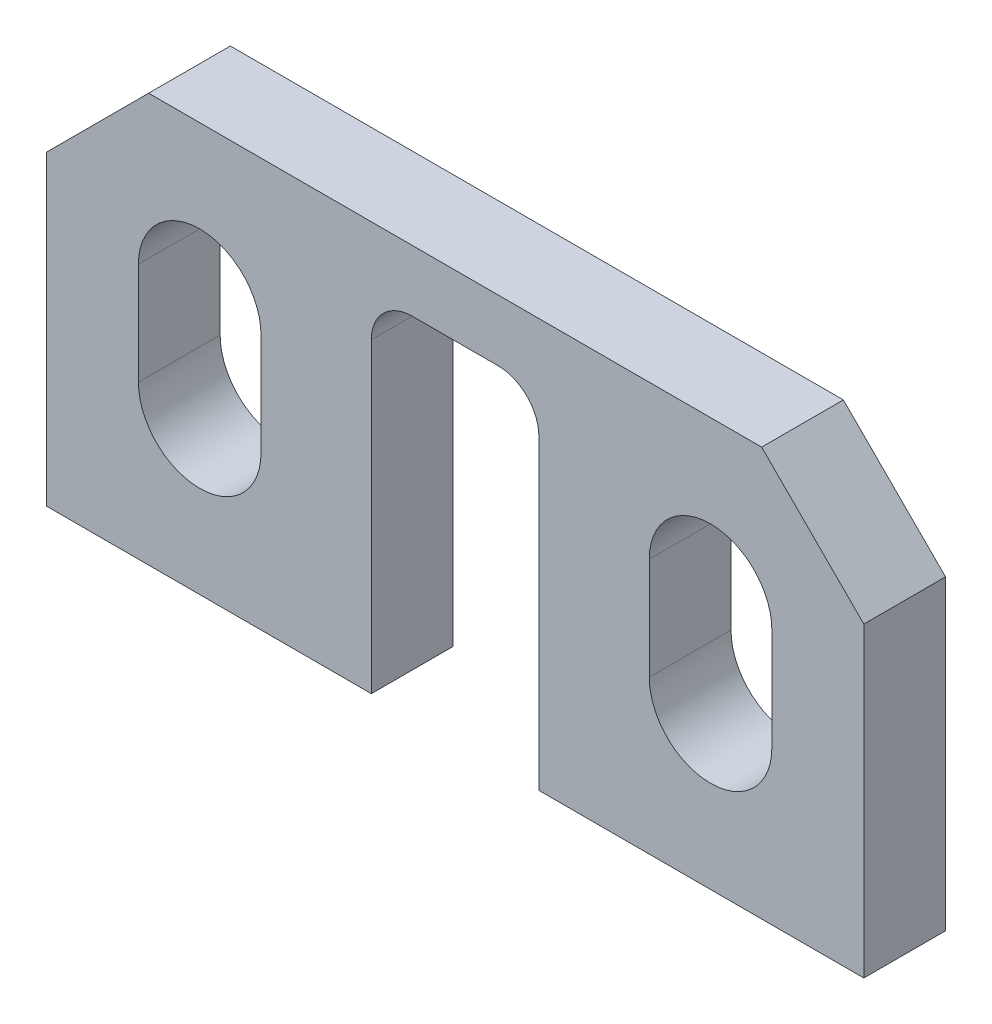
SolidWorks part; units mm, degrees
ref_plane "前视基准面" through (0, 0, 0) normal (0, 0, 1) x (1, 0, 0)
ref_plane "上视基准面" through (0, 0, 0) normal (0, 1, 0) x (1, 0, 0)
ref_plane "右视基准面" through (0, 0, 0) normal (1, 0, 0) x (0, 0, -1)
sketch "草图1" plane through (0, 0, 0) normal (0, 0, 1) x (1, 0, 0)
  line L0 (0, 10) -> (0, 0) construction
  line L1 (-20, 10) -> (20, 10)
  line L2 (-20, 10) -> (-20, -10)
  line L3 (-20, -10) -> (20, -10)
  line L4 (20, 10) -> (20, -10)
  line L5 (0, 0) -> (20, 0) construction
  dimension "D1" = 40
  dimension "D2" = 20
extrude "凸台-拉伸1" add sketch "草图1" along normal blind 4
sketch "草图2" plane through (0, 0, 4) normal (0, 0, 1) x (1, 0, 0)
  line L0 (0, 7) -> (0, -18.9473) construction
  line L1 (4.1, 7) -> (4.1, -18.9473)
  line L2 (-4.1, 7) -> (-4.1, -18.9473)
  line L3 (20, 10) -> (-20, 10) construction
  line L4 (-4.1, 7) -> (4.1, 7)
  arc A1 (-4.1, -18.9473) -> (4.1, -18.9473) centre (0, -18.9473) ccw
  point P3 (0, -7.9736)
  dimension "D1" = 8.2
  dimension "D2" = 3
extrude "切除-拉伸1" cut sketch "草图2" against normal through all
chamfer "倒角1" distance 5 angle 45 2 edges at (20, 10, 2) (-20, 10, 2)
sketch "草图3" plane through (0, 0, 4) normal (0, 0, 1) x (1, 0, 0)
  line L0 (0, 15.5999) -> (0, 0) construction
  line L1 (0, 0) -> (25, 0) construction
  circle A0 centre (-12.5, 0) radius 3
  circle A1 centre (12.5, 0) radius 3
  dimension "D1" = 6
  dimension "D2" = 25
extrude "切除-拉伸2" cut sketch "草图3" against normal through all
sketch "草图5" plane through (0, 0, 4) normal (0, 0, 1) x (1, 0, 0)
  line L0 (-12.5, 2.5) -> (-12.5, -2.5) construction
  line L1 (-9.5, 2.5) -> (-9.5, -2.5)
  line L2 (-15.5, 2.5) -> (-15.5, -2.5)
  arc A0 (-9.5, 2.5) -> (-15.5, 2.5) centre (-12.5, 2.5) ccw
  arc A1 (-15.5, -2.5) -> (-9.5, -2.5) centre (-12.5, -2.5) ccw
  point P2 (-12.5, 0)
  dimension "D1" = 6
  dimension "D2" = 5
extrude "切除-拉伸3" cut sketch "草图5" against normal through all
pattern_linear "阵列(线性)1" count 2 spacing 25 along (1, 0, 0) of "切除-拉伸3"
fillet "圆角1" radius 2 2 edges at (4.1, 7, 2) (-4.1, 7, 2)
sketch "草图6" plane through (0, 0, 4) normal (0, 0, 1) x (1, 0, 0)
  line L0 (-15.5, 0) -> (-9.5, 0) construction
  line L1 (-15.5, 2.5) -> (-15.5, -2.5) construction
  line L2 (-9.5, -2.5) -> (-9.5, 2.5) construction
  line L3 (9.5, 0) -> (15.5, 0) construction
  line L4 (9.5, 2.5) -> (9.5, -2.5) construction
  line L5 (15.5, -2.5) -> (15.5, 2.5) construction
  circle A0 centre (-12.5, 0) radius 3
  circle A1 centre (12.5, 0) radius 3
